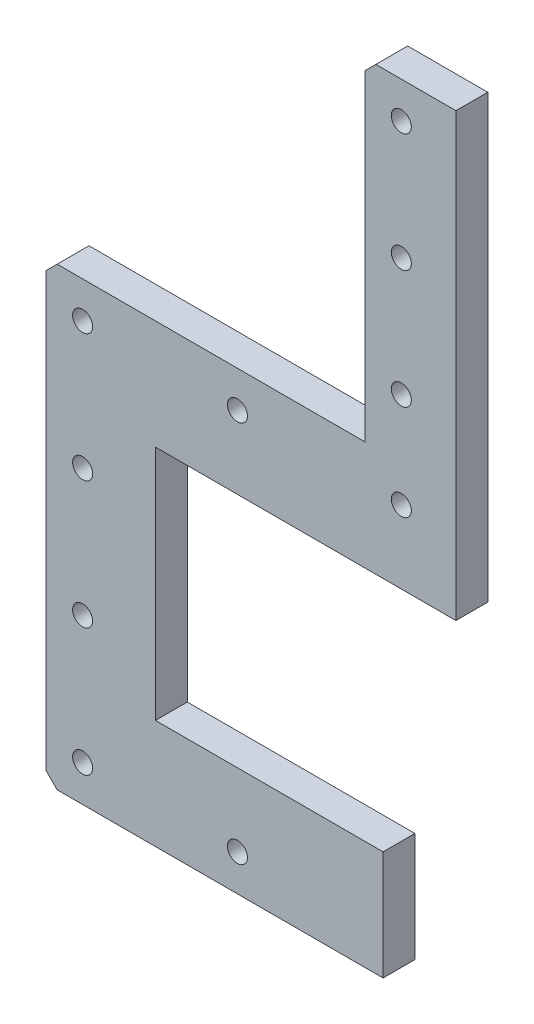
SolidWorks part; units mm, degrees
ref_plane "前视基准面" through (0, 0, 0) normal (0, 0, 1) x (1, 0, 0)
ref_plane "上视基准面" through (0, 0, 0) normal (0, 1, 0) x (1, 0, 0)
ref_plane "右视基准面" through (0, 0, 0) normal (1, 0, 0) x (0, 0, -1)
sketch "草图1" plane through (0, 0, 0) normal (0, 0, 1) x (1, 0, 0)
  line L0 (0, 0) -> (0, -485)
  line L1 (0, 0) -> (-100, 0)
  line L4 (-100, 0) -> (-100, -365)
  line L5 (-450, -365) -> (-450, -865)
  line L6 (-450, -865) -> (-80, -865)
  line L7 (-100, -365) -> (-450, -365)
  line L9 (0, -485) -> (-330, -485)
  line L14 (-330, -485) -> (-330, -745)
  line L17 (-330, -745) -> (-80, -745)
  line L18 (-80, -865) -> (-80, -745)
  line L19 (-80, -895) -> (-80, -745) construction
  dimension "D1" = 365
  dimension "D2" = 500
  dimension "D3" = 100
  dimension "D4" = 120
  dimension "D5" = 120
  dimension "D6" = 120
  dimension "D7" = 450
extrude "凸台-拉伸1" add sketch "草图1" along normal blind 35
chamfer "倒角1" distance 12 angle 45 3 edges at (-450, -865, 17.5) (-450, -365, 17.5) (-100, 0, 17.5)
sketch "草图2" plane through (0, 0, 35) normal (0, 0, 1) x (1, 0, 0)
  line L0 (-60, 0) -> (-60, -485) construction
  line L1 (0, 0) -> (-88, 0) construction
  line L2 (-330, -485) -> (0, -485) construction
  line L3 (0, -405) -> (-450, -405) construction
  line L4 (0, -485) -> (0, 0) construction
  line L5 (-450, -377) -> (-450, -853) construction
  line L6 (-410, -365) -> (-410, -865) construction
  line L7 (-100, -365) -> (-438, -365) construction
  line L8 (-438, -865) -> (-80, -865) construction
  line L9 (-450, -825) -> (-80, -825) construction
  line L10 (-80, -865) -> (-80, -745) construction
  line L11 (-100, -12) -> (-100, -365) construction
  circle A0 centre (-60, -40) radius 11
  circle A1 centre (-60, -170) radius 11
  circle A2 centre (-60, -300) radius 11
  circle A3 centre (-60, -405) radius 11
  circle A4 centre (-240, -405) radius 11
  circle A5 centre (-410, -405) radius 11
  circle A6 centre (-410, -545) radius 11
  circle A7 centre (-410, -685) radius 11
  circle A8 centre (-410, -825) radius 11
  circle A9 centre (-240, -825) radius 11
  dimension "D1" = 22
  dimension "D9" = 140
  dimension "D10" = 40
  dimension "D2" = 40
  dimension "D3" = 130
  dimension "D4" = 130
  dimension "D5" = 170
  dimension "D6" = 105
  dimension "D7" = 140
  dimension "D8" = 140
  dimension "D11" = 170
extrude "切除-拉伸1" cut sketch "草图2" against normal through all both and the other way through all
